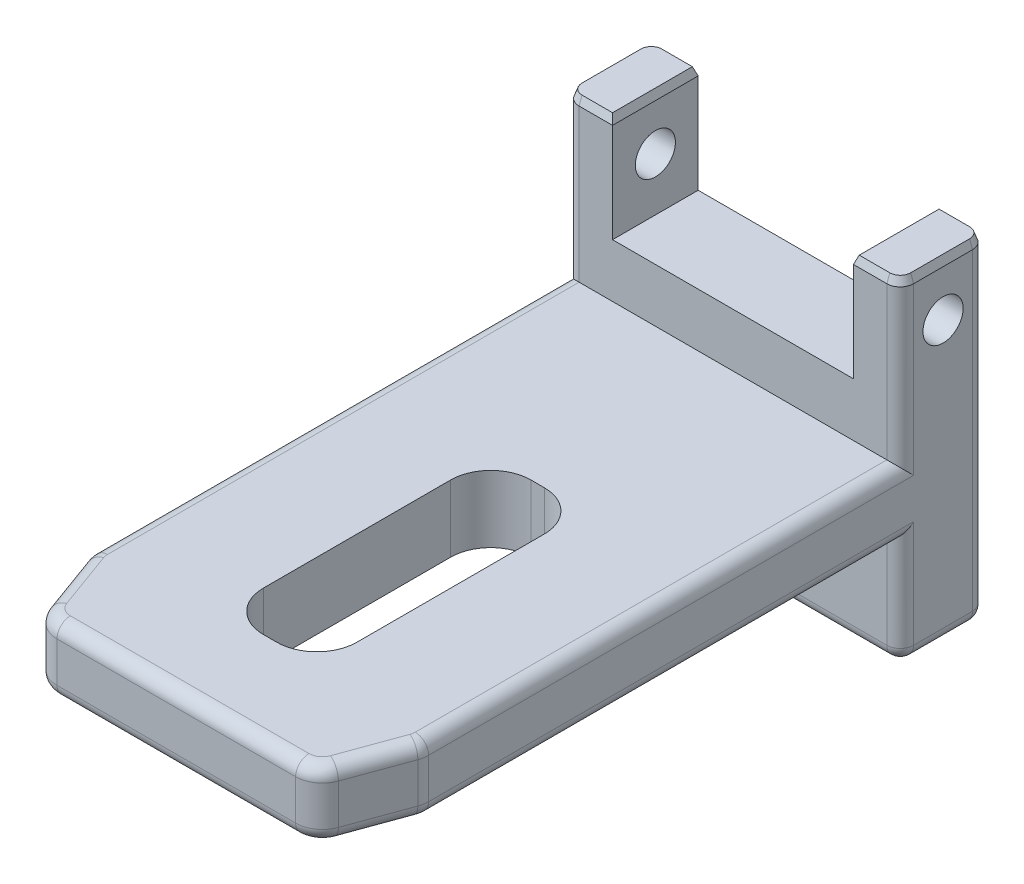
SolidWorks part; units mm, degrees
material "S136H"
ref_plane "Front Plane" through (0, 0, 0) normal (0, 0, 1) x (1, 0, 0)
ref_plane "Top Plane" through (0, 0, 0) normal (0, 1, 0) x (1, 0, 0)
ref_plane "Right Plane" through (0, 0, 0) normal (1, 0, 0) x (0, 0, -1)
sketch "Sketch1" plane through (0, 0, 0) normal (0, 0, 1) x (1, 0, 0)
  line L1 (-6.25, 1.25) -> (6.25, 1.25)
  line L2 (-6.25, 1.25) -> (-6.25, -1.25)
  line L3 (-6.25, -1.25) -> (6.25, -1.25)
  line L4 (6.25, 1.25) -> (6.25, -1.25)
  line L5 (-6.25, 1.25) -> (6.25, -1.25) construction
  line L6 (-6.25, -1.25) -> (6.25, 1.25) construction
  point P0 (0, 0)
  dimension "D1" = 2.5
  dimension "D2" = 12.5
extrude "Boss-Extrude1" add sketch "Sketch1" along normal blind 24
sketch "Sketch2" plane through (0, 1.25, 0) normal (0, 1, 0) x (1, 0, 0)
  line L0 (6.25, -24) -> (6.25, 0) construction
  line L1 (-6.25, 0) -> (6.25, 0)
  line L2 (-6.25, 0) -> (-6.25, -3.2)
  line L3 (-6.25, -3.2) -> (6.25, -3.2)
  line L4 (6.25, 0) -> (6.25, -3.2)
  dimension "D1" = 3.2
extrude "Boss-Extrude2" add sketch "Sketch2" along normal blind 6
sketch "Sketch3" plane through (-6.25, 0, 0) normal (-1, 0, 0) x (0, 0, 1)
  line L0 (24, 1.25) -> (3.2, 1.25) construction
  line L2 (0, 7.25) -> (0, -1.25) construction
  circle A0 centre (1.6, 5.23) radius 0.75
  dimension "D1" = 1.5
  dimension "D2" = 3.98
  dimension "D3" = 1.6
extrude "Cut-Extrude1" cut sketch "Sketch3" against normal blind 13
sketch "Sketch4" plane through (0, 7.25, 0) normal (0, 1, 0) x (1, 0, 0)
  line L0 (-6.25, -3.2) -> (6.25, -3.2) construction
  line L1 (-4.5, 3.2) -> (4.5, 3.2)
  line L2 (-4.5, 3.2) -> (-4.5, -3.2)
  line L3 (-4.5, -3.2) -> (4.5, -3.2)
  line L4 (4.5, 3.2) -> (4.5, -3.2)
  line L5 (-4.5, 3.2) -> (4.5, -3.2) construction
  line L6 (-4.5, -3.2) -> (4.5, 3.2) construction
  point P0 (0, 0)
  dimension "D1" = 9
extrude "Cut-Extrude2" cut sketch "Sketch4" against normal blind 4
sketch "Sketch5" plane through (0, -1.25, 0) normal (0, -1, 0) x (1, 0, 0)
  line L1 (-6.25, 0) -> (6.25, 0)
  line L2 (-6.25, 0) -> (-6.25, 3.2)
  line L3 (-6.25, 3.2) -> (6.25, 3.2)
  line L4 (6.25, 0) -> (6.25, 3.2)
extrude "Boss-Extrude3" add sketch "Sketch5" along normal blind 4
sketch "Sketch7" plane through (0, -1.25, 0) normal (0, -1, 0) x (1, 0, 0)
  line L0 (0, 24) -> (0, 3.2) construction
  line L1 (-6.25, 24) -> (6.25, 24) construction
  line L2 (6.25, 3.2) -> (-6.25, 3.2) construction
  line L4 (-1.75, 20.5) -> (1.75, 20.5)
  line L5 (-1.75, 20.5) -> (-1.75, 10.5)
  line L6 (-1.75, 10.5) -> (1.75, 10.5)
  line L7 (1.75, 20.5) -> (1.75, 10.5)
  line L8 (-1.75, 20.5) -> (1.75, 10.5) construction
  line L9 (-1.75, 10.5) -> (1.75, 20.5) construction
  point P6 (0, 15.5)
  dimension "D1" = 3.5
  dimension "D2" = 3.5
  dimension "D3" = 10
extrude "Cut-Extrude3" cut sketch "Sketch7" against normal blind 4
fillet "Fillet3" radius 1.5 4 edges at (-1.75, 0, 10.5) (-1.75, 0, 20.5) (1.75, 0, 10.5) (1.75, 0, 20.5)
chamfer "Chamfer1" distance 3 angle 20 2 edges at (6.25, 0, 24) (-6.25, 0, 24)
fillet "Fillet1" radius 1 4 edges at (6.25, 0, 21) (5.1581, 0, 24) (-6.25, 0, 21) (-5.1581, 0, 24)
fillet "Fillet2" radius 0.5 28 edges at (-6.25, -1.25, 12.0118) (-6.2348, -1.25, 20.9973) (-5.7936, -1.25, 22.2539) (-5.0315, -1.25, 23.8192) (0, -1.25, 24) (5.0315, -1.25, 23.8192) (5.7936, -1.25, 22.2539) (6.2348, -1.25, 20.9973) (-6.25, 1.25, 12.0118) (-6.2348, 1.25, 20.9973) (-5.7936, 1.25, 22.2539) (6.25, 1.25, 12.0118) (6.2348, 1.25, 20.9973) (5.7936, 1.25, 22.2539) (5.0315, 1.25, 23.8192) (0, 1.25, 24) (6.25, -1.25, 12.0118) (-5.0315, 1.25, 23.8192) (6.25, 4.25, 3.2) (6.25, -3.25, 3.2) (6.25, 1, 0) (-6.25, 4.25, 3.2) (-6.25, 1, 0) (-6.25, -3.25, 3.2) (0, -5.25, 3.2) (6.25, -5.25, 1.6) (0, -5.25, 0) (-6.25, -5.25, 1.6)
chamfer "Chamfer2" distance 0.3 angle 20 12 edges at (4.5, 7.25, 1.6) (5.125, 7.25, 0) (6.1036, 7.25, 0.1464) (6.25, 7.25, 1.6) (6.1036, 7.25, 3.0536) (5.125, 7.25, 3.2) (-4.5, 7.25, 1.6) (-5.125, 7.25, 3.2) (-6.1036, 7.25, 3.0536) (-6.25, 7.25, 1.6) (-6.1036, 7.25, 0.1464) (-5.125, 7.25, 0)
equation "\"code1\"= \"图名分离代码\""
equation "\"code2\"= \"图号分离代码\""
